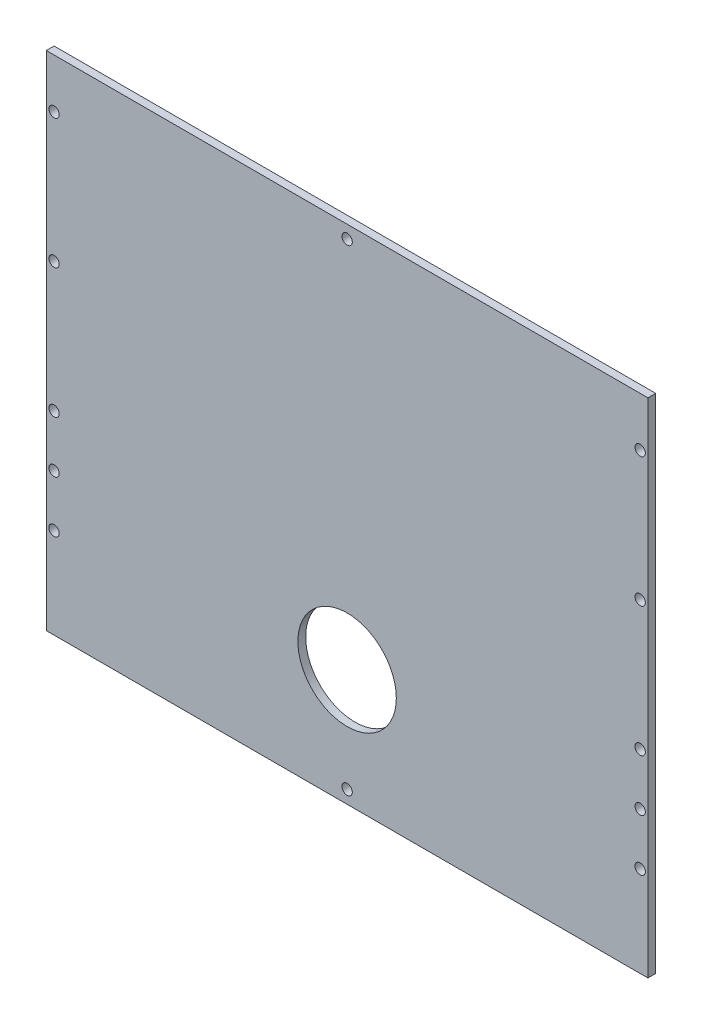
from build123d import *

# Parameters (mm, degrees)
SKETCH1_W           = 232.3
SKETCH1_H           = 194
BOSS_EXTRUDE1_DEPTH = 3
SKETCH2_R           = 19
CUT_EXTRUDE1_DEPTH  = 3
SKETCH3_R           = 2
CUT_EXTRUDE2_DEPTH  = 4
SKETCH4_R           = 2
CUT_EXTRUDE3_DEPTH  = 152.356607058


with BuildPart() as part:
    # Sketch1 → Boss-Extrude1 (new body)
    with BuildSketch(Plane.XY):
        Rectangle(SKETCH1_W, SKETCH1_H)
    extrude(amount=BOSS_EXTRUDE1_DEPTH)

    # Sketch2 → Cut-Extrude1 (cut)
    with BuildSketch(Plane.XY.offset(3)):
        with Locations((0, -52)):
            Circle(SKETCH2_R)
    extrude(amount=-CUT_EXTRUDE1_DEPTH, mode=Mode.SUBTRACT)

    # Sketch3 → Cut-Extrude2 (cut)
    with BuildSketch(Plane.XY.offset(3)):
        with Locations((0, 92)):
            Circle(SKETCH3_R)
        with Locations((0, -92)):
            Circle(SKETCH3_R)
    extrude(amount=-CUT_EXTRUDE2_DEPTH, mode=Mode.SUBTRACT)

    # Sketch4 → Cut-Extrude3 (cut, through all)
    with BuildSketch(Plane.XY.offset(3)):
        with Locations((-113.15, 78)):
            Circle(SKETCH4_R)
        with Locations((-113.15, 28)):
            Circle(SKETCH4_R)
        with Locations((-113.15, -22)):
            Circle(SKETCH4_R)
        with Locations((-113.15, -42)):
            Circle(SKETCH4_R)
        with Locations((-113.15, -62)):
            Circle(SKETCH4_R)
    cut_extrude3 = extrude(amount=-CUT_EXTRUDE3_DEPTH, mode=Mode.SUBTRACT)

    # Mirror1: Cut-Extrude3 across plane
    add(cut_extrude3.mirror(Plane(origin=(0, 0, 0), x_dir=(0, 0, 1), z_dir=(1, 0, 0))), mode=Mode.SUBTRACT)


solid = part.part
